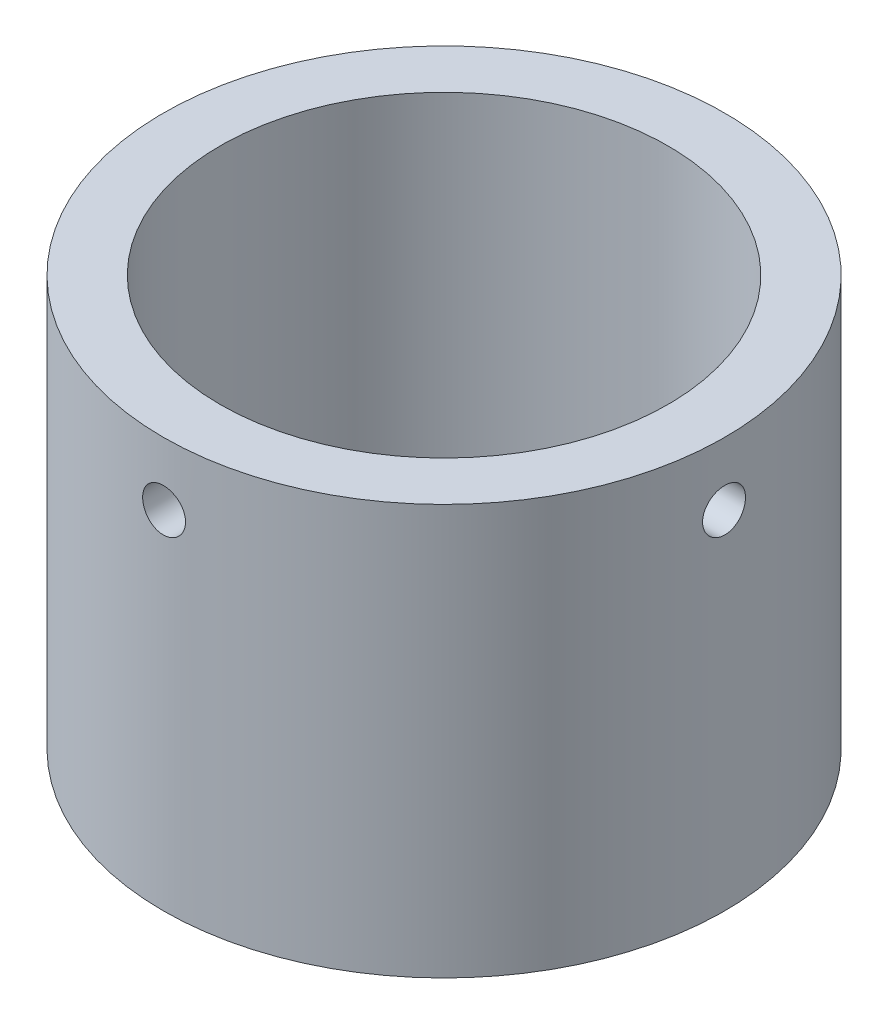
from build123d import *

# Parameters (mm, degrees)
SKETCH1_R           = 44.5
SKETCH1_R_2         = 35.5
BOSS_EXTRUDE1_DEPTH = 65
SKETCH3_R           = 3.4
CUT_EXTRUDE1_DEPTH  = 10
SKETCH4_R           = 3.4
CUT_EXTRUDE2_DEPTH  = 10


with BuildPart() as part:
    # Sketch1 → Boss-Extrude1 (new body)
    with BuildSketch(Plane(origin=(0, 0, 0), x_dir=(1, 0, 0), z_dir=(0, 1, 0))):
        with Locations(Location((0, 0, 0), (0, 0, 270))):
            Circle(SKETCH1_R)
        with Locations(Location((0, 0, 0), (0, 0, 270))):
            Circle(SKETCH1_R_2, mode=Mode.SUBTRACT)
    extrude(amount=BOSS_EXTRUDE1_DEPTH)

    # Sketch3 → Cut-Extrude1 (cut)
    with BuildSketch(Plane(origin=(44.5, 0, 0), x_dir=(0, 0, -1), z_dir=(1, 0, 0))):
        with Locations((0, 55)):
            Circle(SKETCH3_R)
    extrude(amount=-CUT_EXTRUDE1_DEPTH, mode=Mode.SUBTRACT)

    # Sketch4 → Cut-Extrude2 (cut)
    with BuildSketch(Plane.XY.offset(44.5)):
        with Locations((0, 55)):
            Circle(SKETCH4_R)
    extrude(amount=-CUT_EXTRUDE2_DEPTH, mode=Mode.SUBTRACT)


solid = part.part
